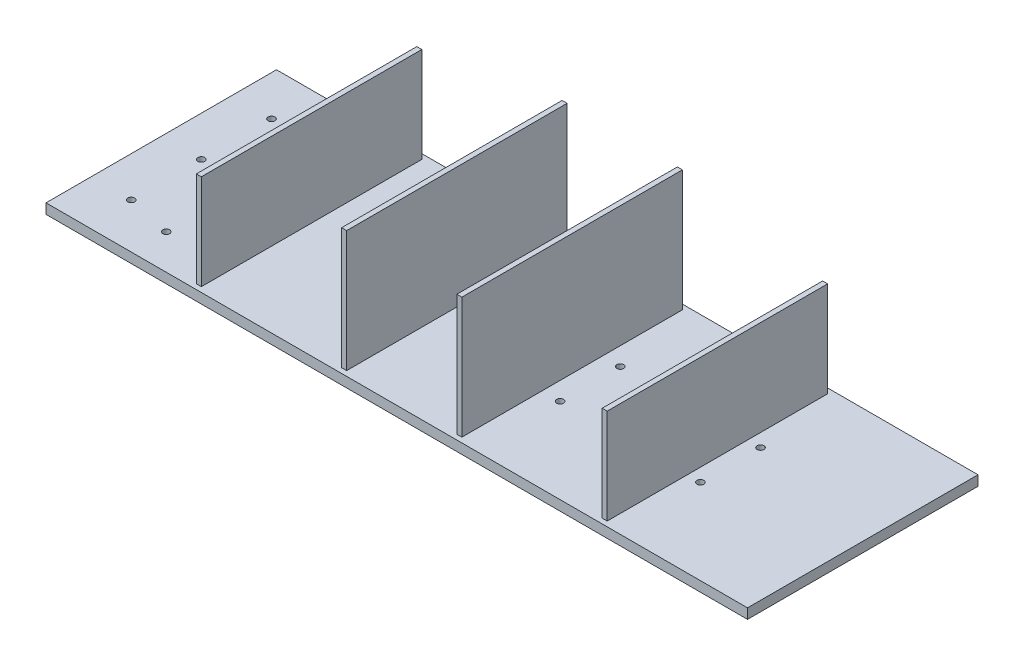
from build123d import *

# Parameters (mm, degrees)
SKETCH1_W             = 700
SKETCH1_H             = 230
BOSS_EXTRUDE1_DEPTH   = 10
M8_TAPPED_HOLE1_D     = 6.8
SKETCH8_W             = 5
SKETCH8_H             = 220
BOSS_EXTRUDE2_DEPTH   = 121
SKETCH9_W             = 5
SKETCH9_H             = 220
BOSS_EXTRUDE3_DEPTH   = 95
M8_TAPPED_HOLE3_D     = 6.8
M8_TAPPED_HOLE3_DEPTH = 19.75
M8_TAPPED_HOLE3_TIP   = 2.042926105


with BuildPart() as part:
    # Sketch1 → Boss-Extrude1 (new body)
    with BuildSketch(Plane(origin=(0, 0, 0), x_dir=(1, 0, 0), z_dir=(0, 1, 0))):
        with Locations((350, -115)):
            Rectangle(SKETCH1_W, SKETCH1_H)
    extrude(amount=BOSS_EXTRUDE1_DEPTH)

    # M8 Tapped Hole1 (through all)
    with Locations(Plane(origin=(0, 10, 0), x_dir=(1, 0, 0), z_dir=(0, 1, 0))):
        with Locations((272, -85), (272, -145), (132, -145), (132, -85), (568, -85), (568, -145), (428, -145), (428, -85)):
            Hole(M8_TAPPED_HOLE1_D / 2)

    # Sketch8 → Boss-Extrude2 (add)
    with BuildSketch(Plane(origin=(0, 10, 0), x_dir=(1, 0, 0), z_dir=(0, 1, 0))):
        with Locations((292.5, -115)):
            Rectangle(SKETCH8_W, SKETCH8_H)
        with Locations((407.5, -115)):
            Rectangle(SKETCH8_W, SKETCH8_H)
    extrude(amount=BOSS_EXTRUDE2_DEPTH)

    # Sketch9 → Boss-Extrude3 (add)
    with BuildSketch(Plane(origin=(0, 10, 0), x_dir=(1, 0, 0), z_dir=(0, 1, 0))):
        with Locations((147.5, -115)):
            Rectangle(SKETCH9_W, SKETCH9_H)
        with Locations((552.5, -115)):
            Rectangle(SKETCH9_W, SKETCH9_H)
    extrude(amount=BOSS_EXTRUDE3_DEPTH)

    # M8 Tapped Hole3
    with Locations(Plane(origin=(0, 0, 0), x_dir=(-1, 0, 0), z_dir=(0, -1, 0))):
        with Locations((-85, -35), (-40, -45), (-40, -185), (-85, -195), (-40, -115), (-85, -115)):
            Hole(M8_TAPPED_HOLE3_D / 2, depth=M8_TAPPED_HOLE3_DEPTH)
            with Locations((0, 0, -(M8_TAPPED_HOLE3_DEPTH + M8_TAPPED_HOLE3_TIP / 2))):  # 118° drill point
                Cone(0, M8_TAPPED_HOLE3_D / 2, M8_TAPPED_HOLE3_TIP, mode=Mode.SUBTRACT)


solid = part.part
